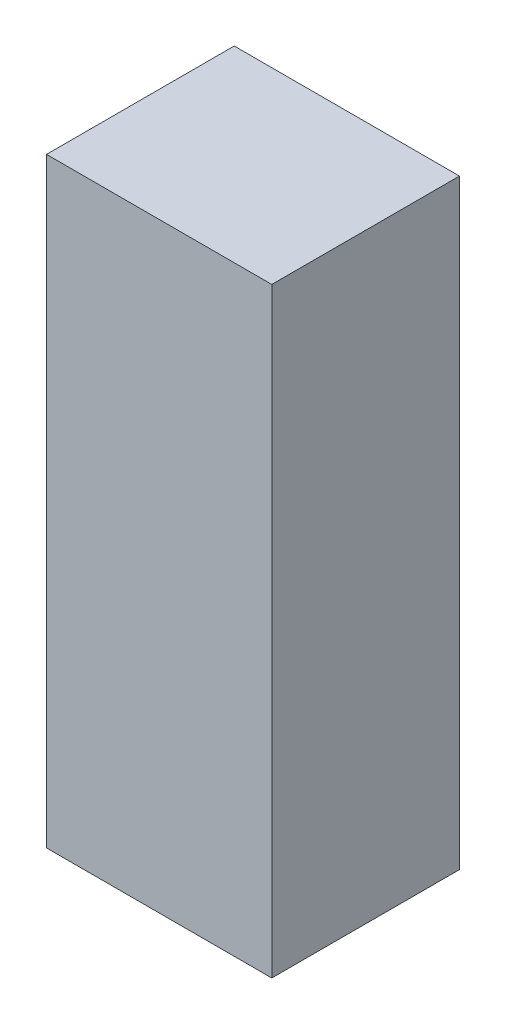
from build123d import *

# Parameters (mm, degrees)
SKETCH_1_W      = 12
SKETCH_1_H      = 32
EXTRUDE_1_DEPTH = 5


with BuildPart() as part:
    # 草图1 → 凸台-拉伸1 (new, symmetric)
    with BuildSketch(Plane.XY):
        Rectangle(SKETCH_1_W, SKETCH_1_H)
    extrude(amount=EXTRUDE_1_DEPTH, both=True)


solid = part.part
